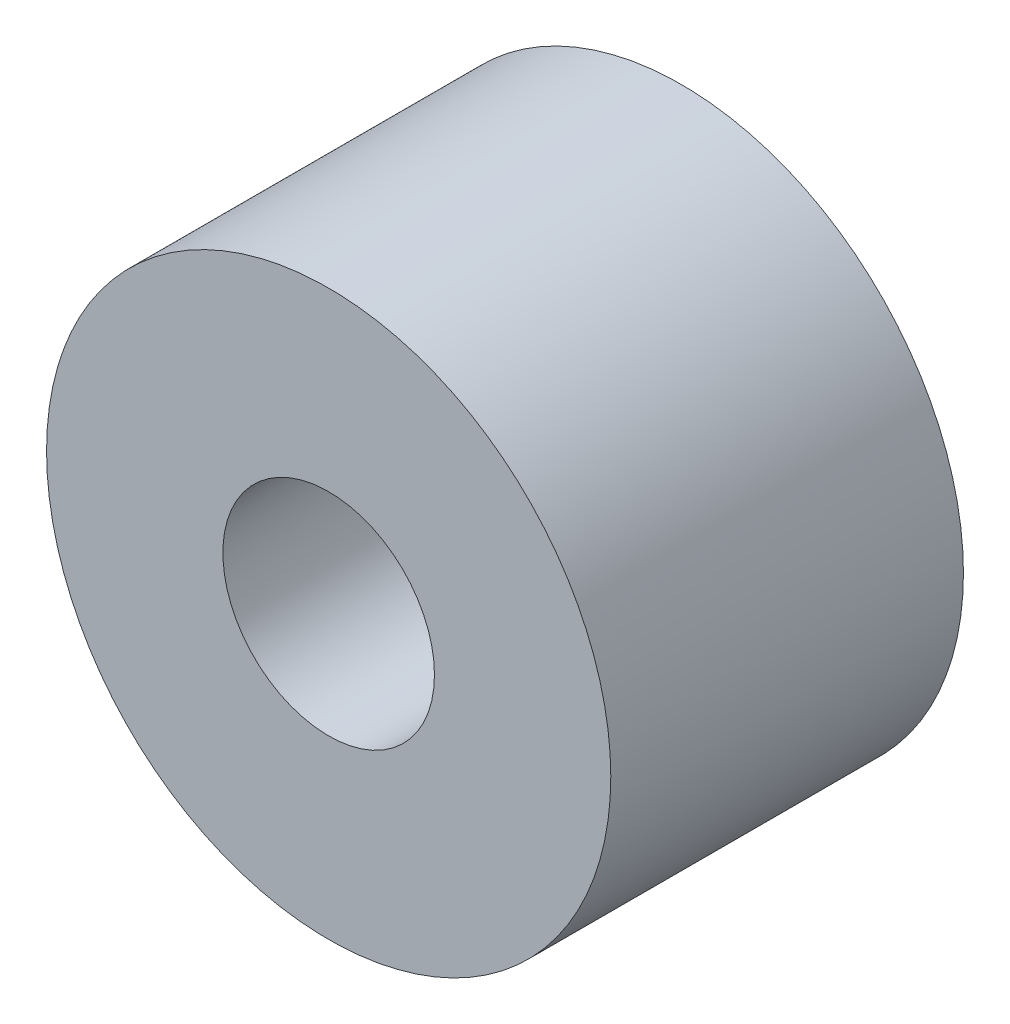
from build123d import *

# Parameters (mm, degrees)
SKETCH_1_R      = 40
SKETCH_1_R_2    = 15
EXTRUDE_1_DEPTH = 50


with BuildPart() as part:
    # 草图1 → 凸台-拉伸1 (new body)
    with BuildSketch(Plane.XY):
        Circle(SKETCH_1_R)
        Circle(SKETCH_1_R_2, mode=Mode.SUBTRACT)
    extrude(amount=EXTRUDE_1_DEPTH)


solid = part.part
